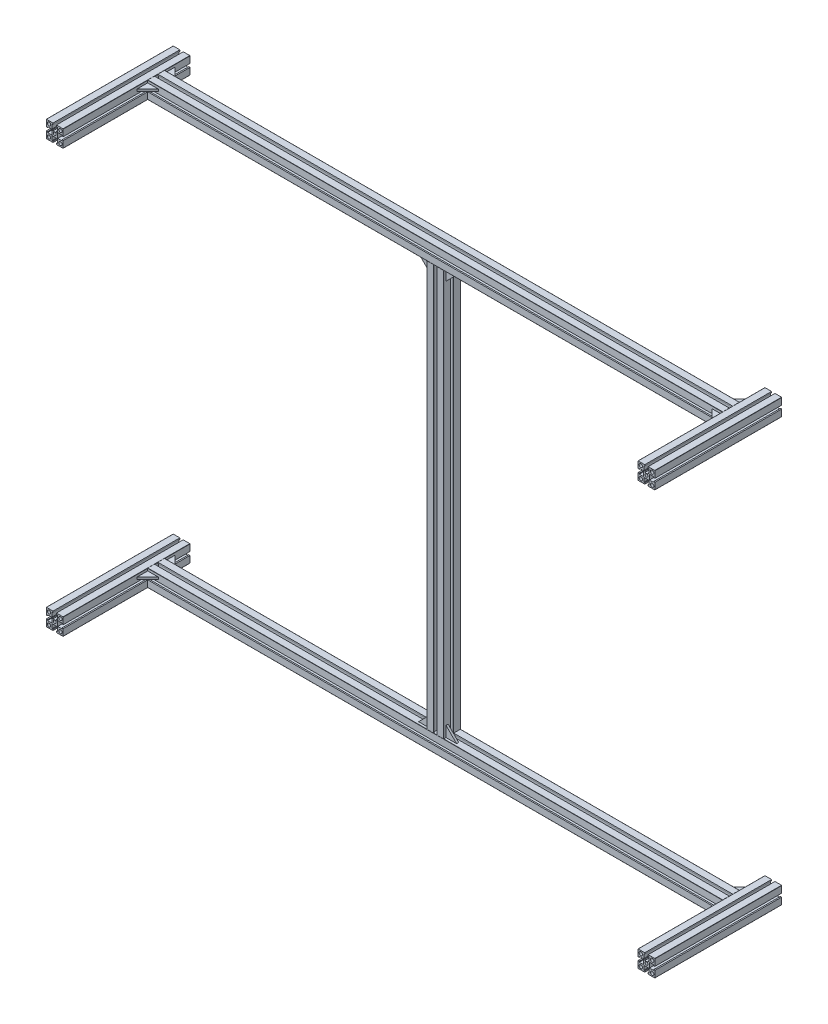
SolidWorks part; units mm, degrees
material "1060 合金"
ref_plane "前视基准面" through (0, 0, 0) normal (0, 0, 1) x (1, 0, 0)
ref_plane "上视基准面" through (0, 0, 0) normal (0, 1, 0) x (1, 0, 0)
ref_plane "右视基准面" through (0, 0, 0) normal (1, 0, 0) x (0, 0, -1)
sketch3d "3D草图1"
  line L13 (-700, 500, 0) -> (700, 500, 0) construction
  line L14 (-700, 500, 0) -> (-700, -500, 0) construction
  line L15 (-700, -500, 0) -> (700, -500, 0) construction
  line L16 (700, 500, 0) -> (700, -500, 0) construction
  line L17 (-700, 500, 0) -> (700, -500, 0) construction
  line L18 (-700, -500, 0) -> (700, 500, 0) construction
  line L22 (-700, 500, 80) -> (-700, -500, 80) construction
  line L23 (700, -500, 80) -> (-700, -500, 80)
  line L24 (700, -500, 80) -> (700, 500, 80) construction
  line L25 (-700, 500, 80) -> (700, 500, 80)
  line L26 (0, 500, 80) -> (0, -500, 80)
  line L27 (-700, 500, 0) -> (-700, 500, 300)
  line L28 (-700, -500, 0) -> (-700, -500, 300)
  line L29 (700, -500, 0) -> (700, -500, 300)
  line L30 (700, 500, 0) -> (700, 500, 300)
  point P0 (0, 0, 0)
  dimension "D1" = 1000
  dimension "D2" = 1400
  dimension "D3" = 300
other "铝型材 40 X 40GF X R0.5(3)"
ref_plane "基准面5" through (-700, 500, 0) normal (0, 0, 1) x (1, 0, 0)
sketch "Sketch1" plane through (-700, 500, 0) normal (0, 0, 1) x (1, 0, 0)
  line L0 (0, 0) -> (0, 20) construction
  line L1 (0, 0) -> (-13.435, 13.435) construction
  line L2 (-19.5, 20) -> (-4, 20)
  line L3 (-20, 19.5) -> (-20, 4)
  line L4 (-19.5, -20) -> (-4, -20)
  line L5 (20, 19.5) -> (20, 4)
  line L6 (-4, 7) -> (-4, 4)
  line L7 (-4, 4) -> (4, 4)
  line L8 (4, 4) -> (4, 7)
  line L9 (0, 0) -> (20, 0) construction
  line L10 (4, 7) -> (6, 7)
  line L11 (13.435, 13.435) -> (0, 0) construction
  line L15 (-4, 20) -> (-4, 17)
  line L20 (-6, 17) -> (-4, 17)
  line L21 (-6, 17) -> (-6, 7)
  line L22 (-6, 7) -> (-4, 7)
  line L23 (6, 17) -> (6, 7)
  line L24 (4, 20) -> (4, 17)
  line L25 (4, 20) -> (19.5, 20)
  line L26 (4, 17) -> (6, 17)
  line L31 (17, 6) -> (7, 6)
  line L32 (17, 6) -> (17, 4)
  line L33 (20, 4) -> (17, 4)
  line L34 (7, 6) -> (7, -6)
  line L35 (17, -6) -> (7, -6)
  line L36 (17, -4) -> (17, -6)
  line L37 (20, -4) -> (17, -4)
  line L38 (6, -17) -> (6, -7)
  line L39 (6, -17) -> (4, -17)
  line L40 (4, -20) -> (4, -17)
  line L41 (6, -7) -> (-6, -7)
  line L42 (-6, -17) -> (-6, -7)
  line L43 (-4, -17) -> (-6, -17)
  line L44 (-4, -20) -> (-4, -17)
  line L45 (-17, -6) -> (-7, -6)
  line L46 (-17, -6) -> (-17, -4)
  line L47 (-20, -4) -> (-17, -4)
  line L48 (-7, -6) -> (-7, 6)
  line L49 (-17, 6) -> (-7, 6)
  line L50 (-17, 4) -> (-17, 6)
  line L51 (-20, 4) -> (-17, 4)
  line L52 (4, -20) -> (19.5, -20)
  line L53 (-20, -4) -> (-20, -19.5)
  line L54 (20, -4) -> (20, -19.5)
  circle A0 centre (0, 0) radius 3.4
  circle A1 centre (-13.435, 13.435) radius 4
  circle A2 centre (13.435, 13.435) radius 4
  circle A3 centre (13.435, -13.435) radius 4
  circle A4 centre (-13.435, -13.435) radius 4
  arc A8 (-19.5, 20) -> (-20, 19.5) centre (-19.5, 19.5) ccw
  arc A9 (19.5, 20) -> (20, 19.5) centre (19.5, 19.5) cw
  arc A10 (19.5, -20) -> (20, -19.5) centre (19.5, -19.5) ccw
  arc A11 (-20, -19.5) -> (-19.5, -20) centre (-19.5, -19.5) ccw
  point P10 (20, -20)
  point P13 (20, 20)
  point P14 (-20, 20)
  point P24 (-20, -20)
  point P25 (0, 0)
  dimension "D2" = 3.4
  dimension "D3" = 45
  dimension "D4" = 8
  dimension "D5" = 3
  dimension "D6" = 19
  dimension "D8" = 12
  dimension "D10" = 10
  dimension "D12" = 40
  dimension "D13" = 8
  dimension "D14" = 0.5
other "角撑板2" parameters "D1"=5, "D2"=5, "D3"=0, "D4"=0, "D10"=5, "D11"=25, "D12"=25, "D13"=15, "D14"=45, "D15"=15
sketch "草图2" plane through (680, 511.75, 100) normal (0, 1, 0) x (1, 0, 0)
  line L0 (0, 0) -> (0, -25)
  line L1 (0, 0) -> (-25, 0)
  line L2 (0, -25) -> (-25, 0)
other "角撑板3" parameters "D1"=5, "D2"=5, "D3"=0, "D4"=0, "D10"=5, "D11"=25, "D12"=25, "D13"=15, "D14"=45, "D15"=15
sketch "草图3" plane through (680, 511.75, 60) normal (0, -1, 0) x (-1, 0, 0)
  line L0 (0, 0) -> (25, 0)
  line L1 (0, 0) -> (0, 25)
  line L2 (25, 0) -> (0, 25)
other "角撑板4" parameters "D1"=5, "D2"=5, "D3"=0, "D4"=0, "D10"=5, "D11"=25, "D12"=25, "D13"=15, "D14"=45, "D15"=15
sketch "草图4" plane through (-20, 480, 91.75) normal (0, 0, -1) x (-1, 0, 0)
  line L0 (0, 0) -> (0, -25)
  line L1 (0, 0) -> (25, 0)
  line L2 (0, -25) -> (25, 0)
other "角撑板5" parameters "D1"=5, "D2"=5, "D3"=0, "D4"=0, "D10"=5, "D11"=25, "D12"=25, "D13"=15, "D14"=45, "D15"=15
sketch "草图5" plane through (20, 480, 91.75) normal (0, 0, 1) x (1, 0, 0)
  line L0 (0, 0) -> (25, 0)
  line L1 (0, 0) -> (0, -25)
  line L2 (25, 0) -> (0, -25)
other "角撑板6" parameters "D1"=5, "D2"=5, "D3"=0, "D4"=0, "D10"=5, "D11"=25, "D12"=25, "D13"=15, "D14"=45, "D15"=15
sketch "草图6" plane through (-20, -480, 91.75) normal (0, 0, 1) x (1, 0, 0)
  line L0 (0, 0) -> (0, 25)
  line L1 (0, 0) -> (-25, 0)
  line L2 (0, 25) -> (-25, 0)
other "角撑板7" parameters "D1"=5, "D2"=5, "D3"=0, "D4"=0, "D10"=5, "D11"=25, "D12"=25, "D13"=15, "D14"=45, "D15"=15
sketch "草图7" plane through (20, -480, 91.75) normal (0, 0, -1) x (-1, 0, 0)
  line L0 (0, 0) -> (-25, 0)
  line L1 (0, 0) -> (0, 25)
  line L2 (-25, 0) -> (0, 25)
other "角撑板8" parameters "D1"=5, "D2"=5, "D3"=0, "D4"=0, "D10"=5, "D11"=25, "D12"=25, "D13"=15, "D14"=45, "D15"=15
sketch "草图8" plane through (-680, 511.75, 100) normal (0, -1, 0) x (-1, 0, 0)
  line L0 (0, 0) -> (-25, 0)
  line L1 (0, 0) -> (0, -25)
  line L2 (-25, 0) -> (0, -25)
other "角撑板9" parameters "D1"=5, "D2"=5, "D3"=0, "D4"=0, "D10"=5, "D11"=25, "D12"=25, "D13"=15, "D14"=45, "D15"=15
sketch "草图9" plane through (-680, 511.75, 60) normal (0, 1, 0) x (1, 0, 0)
  line L0 (0, 0) -> (25, 0)
  line L1 (0, 0) -> (0, 25)
  line L2 (25, 0) -> (0, 25)
other "角撑板12" parameters "D1"=5, "D2"=5, "D3"=0, "D4"=0, "D10"=5, "D11"=25, "D12"=25, "D13"=15, "D14"=45, "D15"=15
sketch "草图12" plane through (680, -488.25, 60) normal (0, -1, 0) x (-1, 0, 0)
  line L0 (0, 0) -> (0, 25)
  line L1 (0, 0) -> (25, 0)
  line L2 (0, 25) -> (25, 0)
other "角撑板13" parameters "D1"=5, "D2"=5, "D3"=0, "D4"=0, "D10"=5, "D11"=25, "D12"=25, "D13"=15, "D14"=45, "D15"=15
sketch "草图13" plane through (680, -511.75, 100) normal (0, 1, 0) x (1, 0, 0)
  line L0 (0, 0) -> (0, -25)
  line L1 (0, 0) -> (-25, 0)
  line L2 (0, -25) -> (-25, 0)
other "角撑板14" parameters "D1"=5, "D2"=5, "D3"=0, "D4"=0, "D10"=5, "D11"=25, "D12"=25, "D13"=15, "D14"=45, "D15"=15
sketch "草图14" plane through (-680, -488.25, 60) normal (0, 1, 0) x (1, 0, 0)
  line L0 (0, 0) -> (25, 0)
  line L1 (0, 0) -> (0, 25)
  line L2 (25, 0) -> (0, 25)
other "角撑板15" parameters "D1"=5, "D2"=5, "D3"=0, "D4"=0, "D10"=5, "D11"=25, "D12"=25, "D13"=15, "D14"=45, "D15"=15
sketch "草图15" plane through (-680, -488.25, 100) normal (0, -1, 0) x (-1, 0, 0)
  line L0 (0, 0) -> (0, -25)
  line L1 (0, 0) -> (-25, 0)
  line L2 (0, -25) -> (-25, 0)
